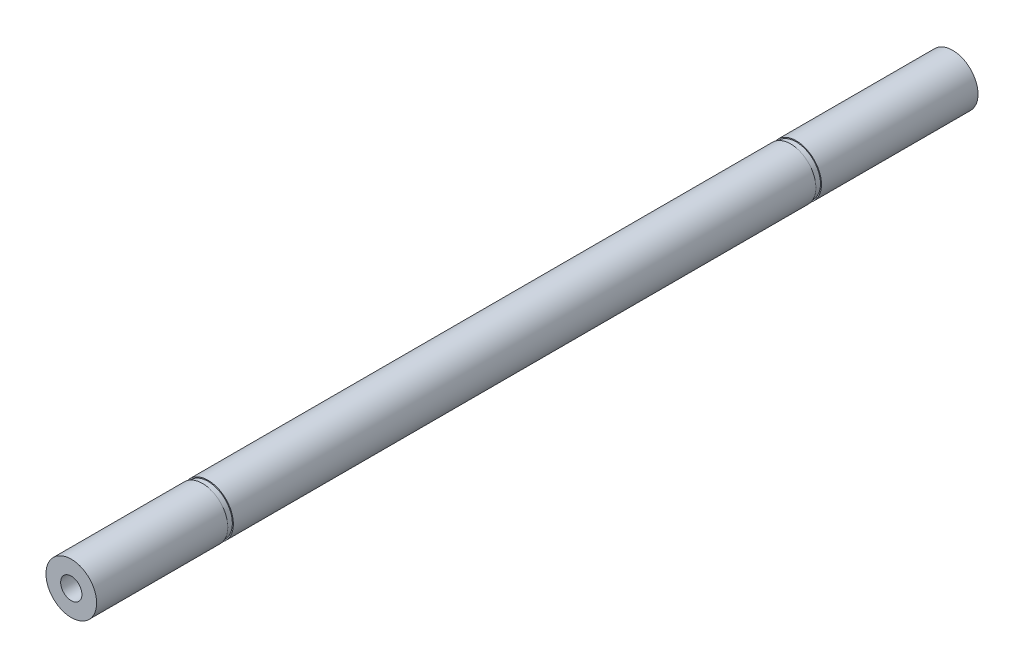
from build123d import *

# Parameters (mm, degrees)
SKETCH1_R             = 5
BOSS_EXTRUDE1_DEPTH   = 87
M5_TAPPED_HOLE1_D     = 4.2
M5_TAPPED_HOLE1_DEPTH = 14
M5_TAPPED_HOLE1_TIP   = 1.2618073
M5_TAPPED_HOLE2_D     = 4.2
M5_TAPPED_HOLE2_DEPTH = 14
M5_TAPPED_HOLE2_TIP   = 1.2618073
SKETCH10_W            = 1.1
SKETCH10_H            = 0.2


with BuildPart() as part:
    # Sketch1 → Boss-Extrude1 (new, symmetric)
    with BuildSketch(Plane.XY):
        Circle(SKETCH1_R)
    extrude(amount=BOSS_EXTRUDE1_DEPTH, both=True)

    # M5 Tapped Hole1
    with Locations(Plane(origin=(0, 0, -87), x_dir=(-1, 0, 0), z_dir=(0, 0, -1))):
        with Locations((0, 0)):
            Hole(M5_TAPPED_HOLE1_D / 2, depth=M5_TAPPED_HOLE1_DEPTH)
            with Locations((0, 0, -(M5_TAPPED_HOLE1_DEPTH + M5_TAPPED_HOLE1_TIP / 2))):  # 118° drill point
                Cone(0, M5_TAPPED_HOLE1_D / 2, M5_TAPPED_HOLE1_TIP, mode=Mode.SUBTRACT)

    # M5 Tapped Hole2
    with Locations(Plane.XY.offset(87)):
        with Locations((0, 0)):
            Hole(M5_TAPPED_HOLE2_D / 2, depth=M5_TAPPED_HOLE2_DEPTH)
            with Locations((0, 0, -(M5_TAPPED_HOLE2_DEPTH + M5_TAPPED_HOLE2_TIP / 2))):  # 118° drill point
                Cone(0, M5_TAPPED_HOLE2_D / 2, M5_TAPPED_HOLE2_TIP, mode=Mode.SUBTRACT)

    # Sketch10 → Cut-Revolve1 (revolve, cut)
    with BuildSketch(Plane(origin=(0, 0, 0), x_dir=(0, 0, -1), z_dir=(1, 0, 0)), mode=Mode.PRIVATE) as cut_revolve1_sk:
        with Locations((-60.55, 4.9)):
            Rectangle(SKETCH10_W, SKETCH10_H)
        with Locations((55.55, 4.9)):
            Rectangle(SKETCH10_W, SKETCH10_H)
    revolve(cut_revolve1_sk.sketch.rotate(Axis((0, 0, 87), (0, 0, -1)), 90), axis=Axis((0, 0, 87), (0, 0, -1)), mode=Mode.SUBTRACT)


solid = part.part
